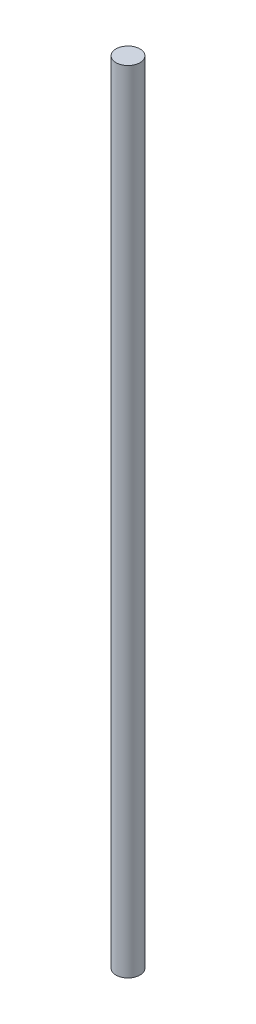
SolidWorks part; units mm, degrees
material "Q235"
ref_plane "Front" through (0, 0, 0) normal (0, 0, 1) x (1, 0, 0)
ref_plane "Top" through (0, 0, 0) normal (0, 1, 0) x (1, 0, 0)
ref_plane "Right" through (0, 0, 0) normal (1, 0, 0) x (0, 0, -1)
sketch "Sketch1" plane through (0, 0, 0) normal (0, 1, 0) x (1, 0, 0)
  circle A0 centre (0, 0) radius 10
  dimension "D1" = 20
extrude "Boss-Extrude1" add sketch "Sketch1" along normal blind 660
